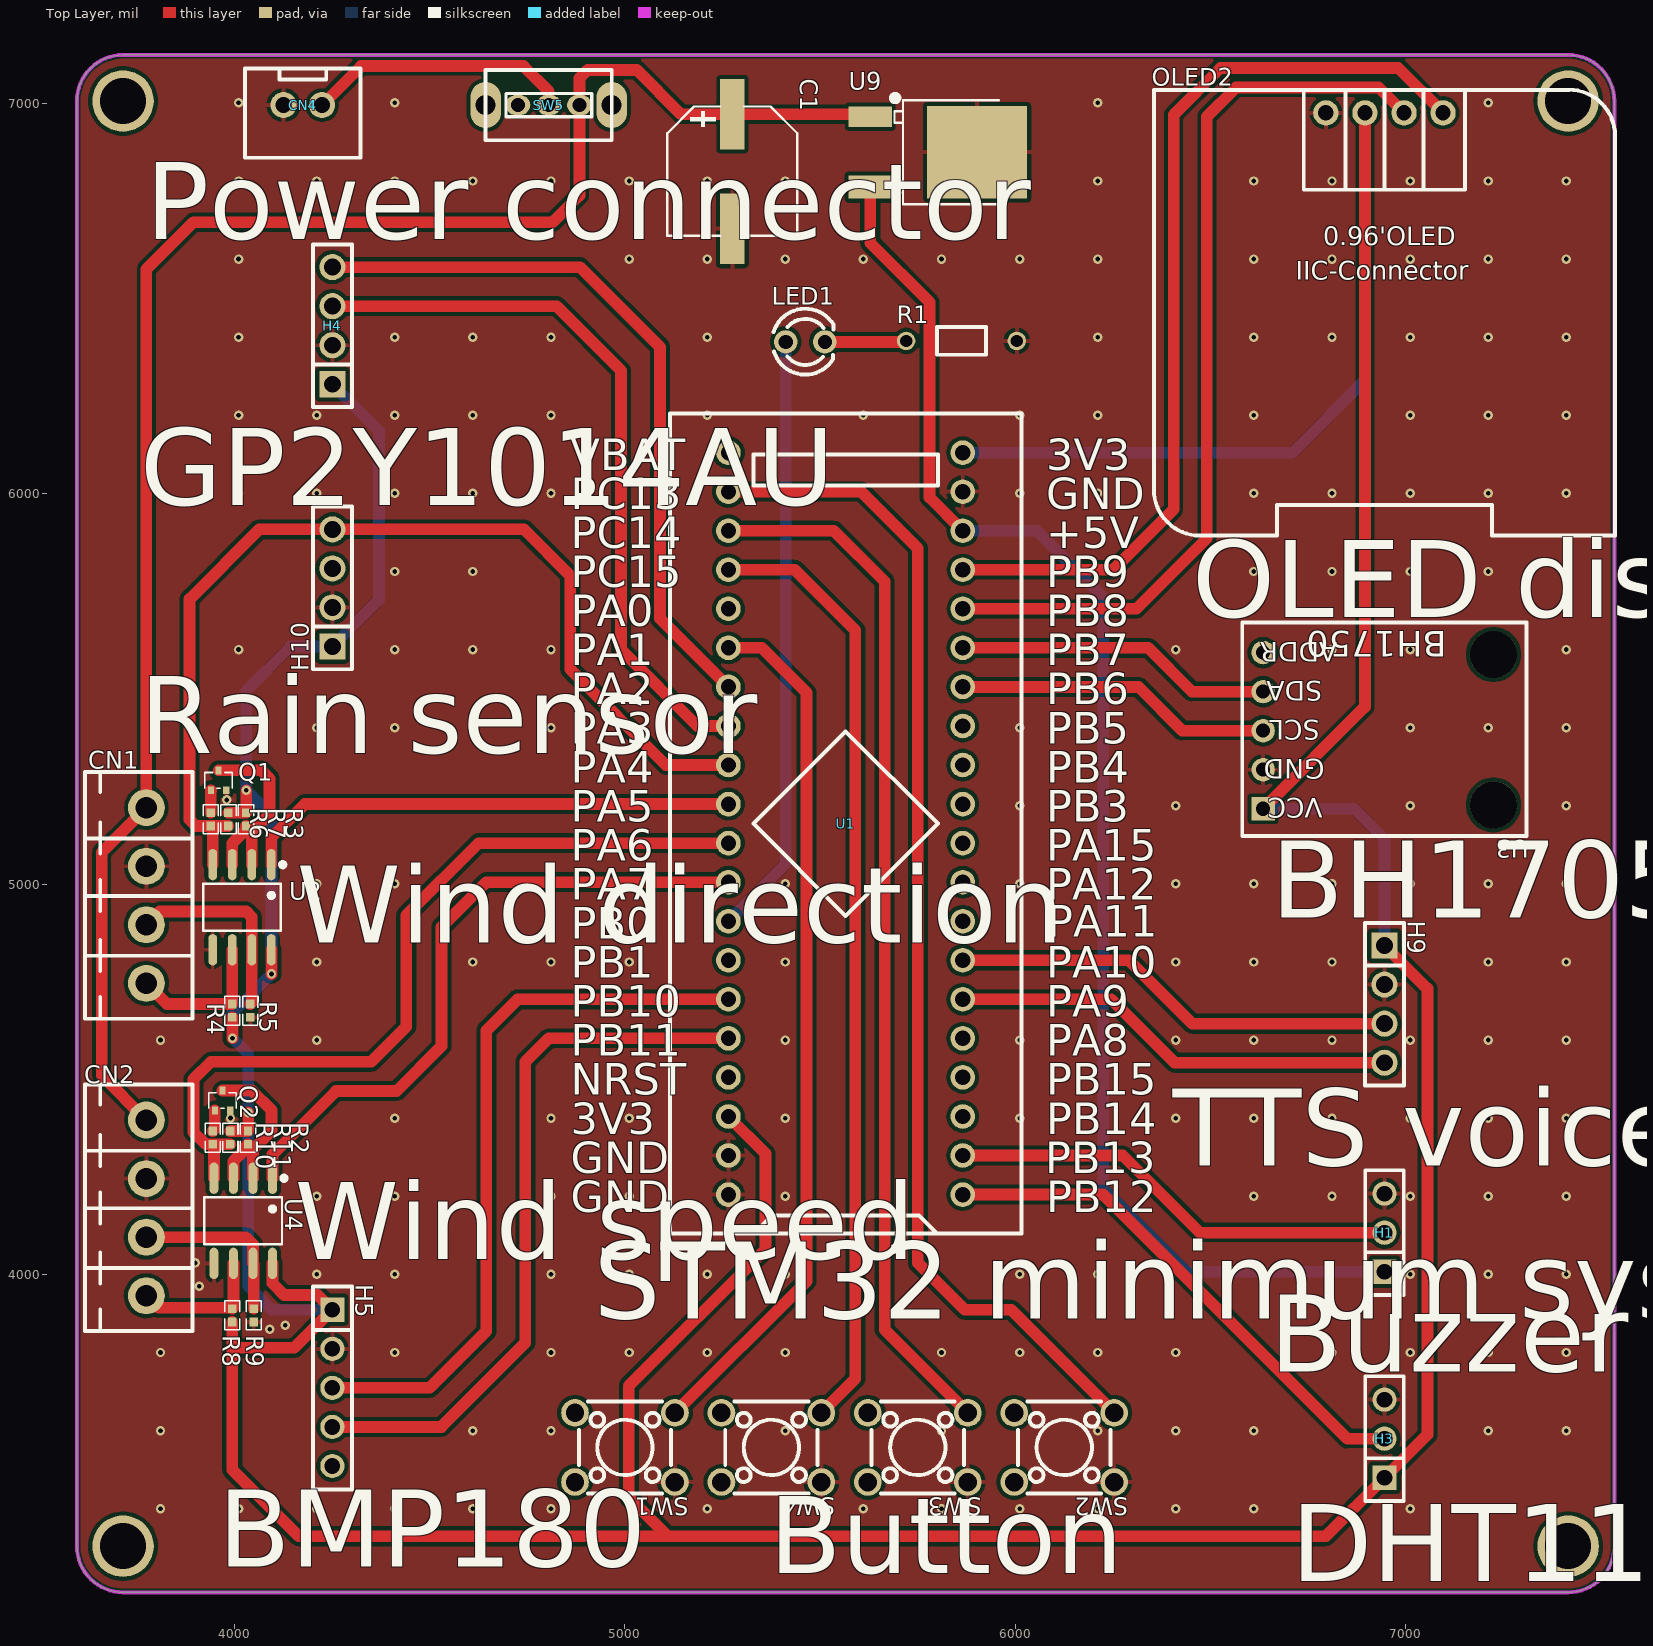
[diagram p0: Top Layer view]
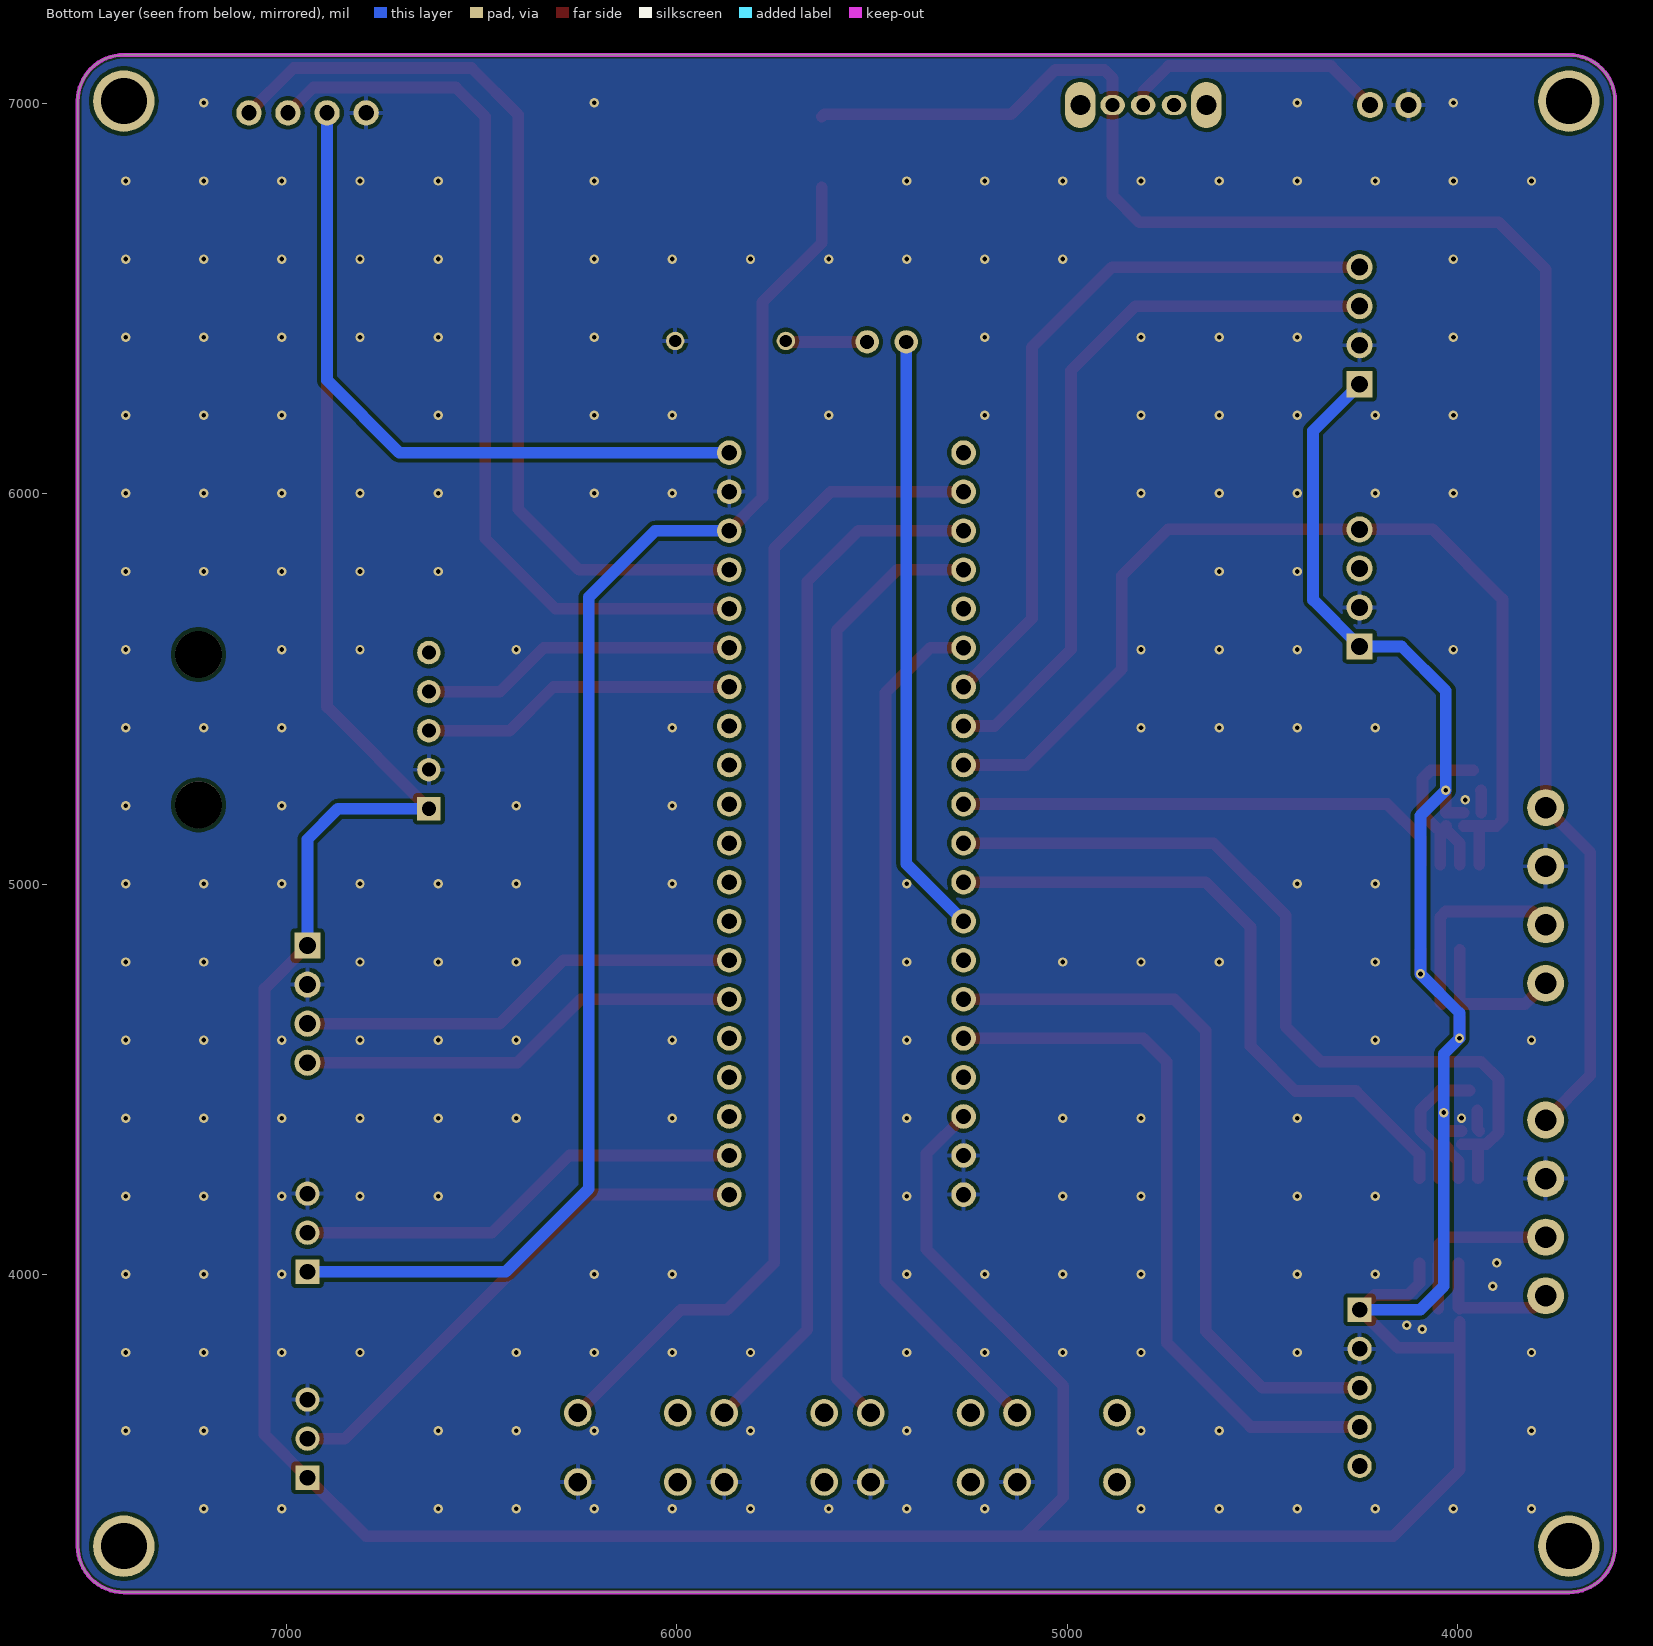
[diagram p1: Bottom Layer view, seen from below]
# Altium PCB MISC51967.pcbdoc
Units mil, origin at the board's own origin, x right, y up, seen from the top; angles counter-clockwise.
Board outline 3937.01 x 3937.01 mil, 2 copper layers (Top Layer, Bottom Layer), stack 62.206 mil thick; 35 components, 48 nets, 160 pads, 207 vias.

## Layer stack, top to bottom
Top Solder Mask Layer: solder mask 0.394, Dk 3.3
Top Layer: signal copper 1.379
Dielectric1: surface 59.449, FR4, Dk 4.5
Bottom Layer: signal copper 1.378
Bottom Solder Mask Layer: solder mask 0.394, Dk 3.3

## Board outline
3714.61,7123.5 ccw(c3714.61,7005.39) 3596.5,7005.39 3596.5,3304.61 ccw(c3714.61,3304.61) 3714.61,3186.5 7415.39,3186.5 ccw(c7415.39,3304.61) 7533.5,3304.61 7533.5,7005.39 ccw(c7415.39,7005.39) 7415.39,7123.5 3714.61,7123.5

## Design rules (kind name [scope] priority, off if disabled: settings)
BoardOutlineClearance copperThickness2oz_1 [All] p2 off: genericclearance=7.99 ignorepadtopadclearanceinfootprint=FALSE except(0: Arc-SplitContinuation Track-SplitContinuation SMDPad-SplitContinuation THPad-SplitContinuation Via-SplitContinuation Fill-SplitContinuation Region-SplitContinuation Poly-SplitContinuation Text-SplitContinuation Hole-SplitContinuation; 5.98: Arc-CutoutEdge Track-CutoutEdge SMDPad-CutoutEdge THPad-CutoutEdge Via-CutoutEdge Text-CutoutEdge; 6.9: Hole-OutlineEdge Hole-CutoutEdge; 10: Poly-OutlineEdge Poly-CutoutEdge; 11.81: Arc-OutlineEdge Track-OutlineEdge SMDPad-OutlineEdge THPad-OutlineEdge Via-OutlineEdge Fill-OutlineEdge Region-OutlineEdge Text-OutlineEdge Fill-CutoutEdge Region-CutoutEdge)
BoardOutlineClearance Plane_innerPlane_1 [All] p4 off: genericclearance=4.02 ignorepadtopadclearanceinfootprint=FALSE except(0: Arc-SplitContinuation Track-SplitContinuation SMDPad-SplitContinuation THPad-SplitContinuation Via-SplitContinuation Fill-SplitContinuation Region-SplitContinuation Poly-SplitContinuation Text-SplitContinuation Hole-SplitContinuation; 5.98: Arc-CutoutEdge Track-CutoutEdge SMDPad-CutoutEdge THPad-CutoutEdge Via-CutoutEdge Text-CutoutEdge; 6.9: Hole-OutlineEdge Hole-CutoutEdge; 10: Poly-OutlineEdge Poly-CutoutEdge; 11.81: Arc-OutlineEdge Track-OutlineEdge SMDPad-OutlineEdge THPad-OutlineEdge Via-OutlineEdge Fill-OutlineEdge Region-OutlineEdge Text-OutlineEdge Fill-CutoutEdge Region-CutoutEdge)
BoardOutlineClearance Copper_copperRegion_1 [All] p6 off: genericclearance=4.02 ignorepadtopadclearanceinfootprint=FALSE except(0: Arc-SplitContinuation Track-SplitContinuation SMDPad-SplitContinuation THPad-SplitContinuation Via-SplitContinuation Fill-SplitContinuation Region-SplitContinuation Poly-SplitContinuation Text-SplitContinuation Hole-SplitContinuation; 5.98: Arc-CutoutEdge Track-CutoutEdge SMDPad-CutoutEdge THPad-CutoutEdge Via-CutoutEdge Text-CutoutEdge; 6.9: Hole-OutlineEdge Hole-CutoutEdge; 10: Poly-OutlineEdge Poly-CutoutEdge; 11.81: Arc-OutlineEdge Track-OutlineEdge SMDPad-OutlineEdge THPad-OutlineEdge Via-OutlineEdge Fill-OutlineEdge Region-OutlineEdge Text-OutlineEdge Fill-CutoutEdge Region-CutoutEdge)
BoardOutlineClearance Copper_copperRegion_copperThickness1oz_1 [All] p8 off: genericclearance=4.02 ignorepadtopadclearanceinfootprint=FALSE except(0: Arc-SplitContinuation Track-SplitContinuation SMDPad-SplitContinuation THPad-SplitContinuation Via-SplitContinuation Fill-SplitContinuation Region-SplitContinuation Poly-SplitContinuation Text-SplitContinuation Hole-SplitContinuation; 5.98: Arc-CutoutEdge Track-CutoutEdge SMDPad-CutoutEdge THPad-CutoutEdge Via-CutoutEdge Text-CutoutEdge; 6.9: Hole-OutlineEdge Hole-CutoutEdge; 10: Poly-OutlineEdge Poly-CutoutEdge; 11.81: Arc-OutlineEdge Track-OutlineEdge SMDPad-OutlineEdge THPad-OutlineEdge Via-OutlineEdge Fill-OutlineEdge Region-OutlineEdge Text-OutlineEdge Fill-CutoutEdge Region-CutoutEdge)
BoardOutlineClearance Copper_copperRegion_Copper_copperRegion_1 [All] p10 off: genericclearance=4.02 ignorepadtopadclearanceinfootprint=FALSE except(0: Arc-SplitContinuation Track-SplitContinuation SMDPad-SplitContinuation THPad-SplitContinuation Via-SplitContinuation Fill-SplitContinuation Region-SplitContinuation Poly-SplitContinuation Text-SplitContinuation Hole-SplitContinuation; 5.98: Arc-CutoutEdge Track-CutoutEdge SMDPad-CutoutEdge THPad-CutoutEdge Via-CutoutEdge Text-CutoutEdge; 6.9: Hole-OutlineEdge Hole-CutoutEdge; 10: Poly-OutlineEdge Poly-CutoutEdge; 11.81: Arc-OutlineEdge Track-OutlineEdge SMDPad-OutlineEdge THPad-OutlineEdge Via-OutlineEdge Fill-OutlineEdge Region-OutlineEdge Text-OutlineEdge Fill-CutoutEdge Region-CutoutEdge)
BoardOutlineClearance copperThickness1oz_1 [All] p12: genericclearance=4.02 ignorepadtopadclearanceinfootprint=FALSE except(0: Arc-SplitContinuation Track-SplitContinuation SMDPad-SplitContinuation THPad-SplitContinuation Via-SplitContinuation Fill-SplitContinuation Region-SplitContinuation Poly-SplitContinuation Text-SplitContinuation Hole-SplitContinuation; 5.98: Arc-CutoutEdge Track-CutoutEdge SMDPad-CutoutEdge THPad-CutoutEdge Via-CutoutEdge Text-CutoutEdge; 6.9: Hole-OutlineEdge Hole-CutoutEdge; 10: Poly-OutlineEdge Poly-CutoutEdge; 11.81: Arc-OutlineEdge Track-OutlineEdge SMDPad-OutlineEdge THPad-OutlineEdge Via-OutlineEdge Fill-OutlineEdge Region-OutlineEdge Text-OutlineEdge Fill-CutoutEdge Region-CutoutEdge)
Clearance copperThickness2oz [All] p1 off: gap=7.99 ignorepadtopadclearanceinfootprint=FALSE except(5.98: SMDPad-Track SMDPad-SMDPad THPad-Track SMDPad-THPad THPad-THPad Track-Via SMDPad-Via THPad-Via Via-Via Fill-SMDPad Region-SMDPad Fill-THPad Region-THPad Fill-Via Region-Via Fill-Fill Fill-Region Region-Region Arc-Track Arc-SMDPad Arc-THPad Arc-Via Fill-Arc Region-Arc Arc-Arc Text-Track SMDPad-Text Text-THPad Text-Via Fill-Text Region-Text Arc-Text Text-Text; 6.9: Hole-Track Hole-SMDPad Hole-THPad Hole-Via Fill-Hole Region-Hole Hole-Arc Hole-Text; 10: Poly-Track Poly-SMDPad Poly-THPad Poly-Via Poly-Fill Poly-Region Poly-Poly Poly-Arc Poly-Text Poly-Hole; 11.81: Fill-Track Region-Track)
Clearance Plane_innerPlane [All] p3 off: gap=4.02 ignorepadtopadclearanceinfootprint=FALSE except(5.98: SMDPad-Track SMDPad-SMDPad THPad-Track SMDPad-THPad THPad-THPad Track-Via SMDPad-Via THPad-Via Via-Via Fill-SMDPad Region-SMDPad Fill-THPad Region-THPad Fill-Via Region-Via Fill-Fill Fill-Region Region-Region Arc-Track Arc-SMDPad Arc-THPad Arc-Via Fill-Arc Region-Arc Arc-Arc Text-Track SMDPad-Text Text-THPad Text-Via Fill-Text Region-Text Arc-Text Text-Text; 6.9: Hole-Track Hole-SMDPad Hole-THPad Hole-Via Fill-Hole Region-Hole Hole-Arc Hole-Text; 10: Poly-Track Poly-SMDPad Poly-THPad Poly-Via Poly-Fill Poly-Region Poly-Poly Poly-Arc Poly-Text Poly-Hole; 11.81: Fill-Track Region-Track)
Clearance Copper_copperRegion [All] p5 off: gap=4.02 ignorepadtopadclearanceinfootprint=FALSE except(5.98: SMDPad-Track SMDPad-SMDPad THPad-Track SMDPad-THPad THPad-THPad Track-Via SMDPad-Via THPad-Via Via-Via Fill-SMDPad Region-SMDPad Fill-THPad Region-THPad Fill-Via Region-Via Fill-Fill Fill-Region Region-Region Arc-Track Arc-SMDPad Arc-THPad Arc-Via Fill-Arc Region-Arc Arc-Arc Text-Track SMDPad-Text Text-THPad Text-Via Fill-Text Region-Text Arc-Text Text-Text; 6.9: Hole-Track Hole-SMDPad Hole-THPad Hole-Via Fill-Hole Region-Hole Hole-Arc Hole-Text; 10: Poly-Track Poly-SMDPad Poly-THPad Poly-Via Poly-Fill Poly-Region Poly-Poly Poly-Arc Poly-Text Poly-Hole; 11.81: Fill-Track Region-Track)
Clearance Copper_copperRegion_copperThickness1oz [All] p7 off: gap=4.02 ignorepadtopadclearanceinfootprint=FALSE except(5.98: SMDPad-Track SMDPad-SMDPad THPad-Track SMDPad-THPad THPad-THPad Track-Via SMDPad-Via THPad-Via Via-Via Fill-SMDPad Region-SMDPad Fill-THPad Region-THPad Fill-Via Region-Via Fill-Fill Fill-Region Region-Region Arc-Track Arc-SMDPad Arc-THPad Arc-Via Fill-Arc Region-Arc Arc-Arc Text-Track SMDPad-Text Text-THPad Text-Via Fill-Text Region-Text Arc-Text Text-Text; 6.9: Hole-Track Hole-SMDPad Hole-THPad Hole-Via Fill-Hole Region-Hole Hole-Arc Hole-Text; 10: Poly-Track Poly-SMDPad Poly-THPad Poly-Via Poly-Fill Poly-Region Poly-Poly Poly-Arc Poly-Text Poly-Hole; 11.81: Fill-Track Region-Track)
Clearance Copper_copperRegion_Copper_copperRegion [All] p9 off: gap=4.02 ignorepadtopadclearanceinfootprint=FALSE except(5.98: SMDPad-Track SMDPad-SMDPad THPad-Track SMDPad-THPad THPad-THPad Track-Via SMDPad-Via THPad-Via Via-Via Fill-SMDPad Region-SMDPad Fill-THPad Region-THPad Fill-Via Region-Via Fill-Fill Fill-Region Region-Region Arc-Track Arc-SMDPad Arc-THPad Arc-Via Fill-Arc Region-Arc Arc-Arc Text-Track SMDPad-Text Text-THPad Text-Via Fill-Text Region-Text Arc-Text Text-Text; 6.9: Hole-Track Hole-SMDPad Hole-THPad Hole-Via Fill-Hole Region-Hole Hole-Arc Hole-Text; 10: Poly-Track Poly-SMDPad Poly-THPad Poly-Via Poly-Fill Poly-Region Poly-Poly Poly-Arc Poly-Text Poly-Hole; 11.81: Fill-Track Region-Track)
Clearance copperThickness1oz [All] p11: gap=4.02 ignorepadtopadclearanceinfootprint=FALSE except(5.98: SMDPad-Track SMDPad-SMDPad THPad-Track SMDPad-THPad THPad-THPad Track-Via SMDPad-Via THPad-Via Via-Via Fill-SMDPad Region-SMDPad Fill-THPad Region-THPad Fill-Via Region-Via Fill-Fill Fill-Region Region-Region Arc-Track Arc-SMDPad Arc-THPad Arc-Via Fill-Arc Region-Arc Arc-Arc Text-Track SMDPad-Text Text-THPad Text-Via Fill-Text Region-Text Arc-Text Text-Text; 6.9: Hole-Track Hole-SMDPad Hole-THPad Hole-Via Fill-Hole Region-Hole Hole-Arc Hole-Text; 10: Poly-Track Poly-SMDPad Poly-THPad Poly-Via Poly-Fill Poly-Region Poly-Poly Poly-Arc Poly-Text Poly-Hole; 11.81: Fill-Track Region-Track)
DiffPairsRouting differentialPair [All] p1: maxlimit=6 minlimit=6 mostfreqgap=6 toplayer_minwidth=5 toplayer_prefwidth=10 toplayer_maxwidth=100 toplayer_mingap=6 toplayer_prefgap=6 toplayer_maxgap=6 bottomlayer_minwidth=5 bottomlayer_prefwidth=10 bottomlayer_maxwidth=100 bottomlayer_mingap=6 bottomlayer_prefgap=6 bottomlayer_maxgap=6 maxuncoupledlength=10
HoleToHoleClearance otherClearance [All] p1: gap=11.81 allowstackedmicrovias=TRUE
Length netLength [All] p1: minlimit=0 maxlimit=0
PasteMaskExpansion pasteMaskExpansion [All] p1: expansion=0
PlaneConnect innerPlane [All] p1: planeconnectstyle=Relief reliefexpansion=20 reliefentries=4 reliefconductorwidth=10 reliefairgap=10
PolygonConnect copperRegion_copperThickness1oz [All] p1 off: connectstyle=Relief reliefconductorwidth=10 reliefentries=4 polygonreliefangle="90 Angle" airgapwidth=10 via.connectstyle=Relief via.reliefconductorwidth=10 via.reliefentries=4 via.polygonreliefangle="90 Angle" via.airgapwidth=10
PolygonConnect copperRegion_Copper_copperRegion [All] p2 off: connectstyle=Relief reliefconductorwidth=10 reliefentries=4 polygonreliefangle="90 Angle" airgapwidth=10 via.connectstyle=Relief via.reliefconductorwidth=10 via.reliefentries=4 via.polygonreliefangle="90 Angle" via.airgapwidth=10
PolygonConnect copperRegion [All] p3: connectstyle=Relief reliefconductorwidth=10 reliefentries=4 polygonreliefangle="90 Angle" airgapwidth=10 via.connectstyle=Relief via.reliefconductorwidth=10 via.reliefentries=4 via.polygonreliefangle="90 Angle" via.airgapwidth=10
RoutingVias viaSize [All] p1: holewidth=12.01 width=24.02 viastyle="Through Hole" minholewidth=11.81 minwidth=19.68 maxholewidth=248.03 maxwidth=393.7
SolderMaskExpansion solderMaskExpansion [IsVia] p1: expansion=-1000 istentingtop=TRUE
SolderMaskExpansion solderMaskExpansion [All] p2: expansion=2 istentingtop=FALSE
Width copperThickness2oz_2 [All] p1 off: maxlimit=100 minlimit=8 preferedwidth=10
Width copperThickness1oz_2 [All] p2: maxlimit=100 minlimit=5 preferedwidth=10

## Components (designator, comment, footprint, x,y, rotation, side; value= is the part's Value field where it differs from the comment)
C1 "" CAP-SMD_BD8.0-L8.3-W8.3-LS9.3-FD 5275,6825 r270 top
CN1 "KF2EDGV-3.81-4P" CONN-TH_4P-P3.81_KF2EDGV-3.81-4P 3774.44,4970.87 r270 top
CN2 "KF2EDGV-3.81-4P" CONN-TH_4P-P3.81_KF2EDGV-3.81-4P 3774.44,4170.87 r270 top
CN4 "XH2.54*2P_through-hole" CONN-TH_2P-P2.50-XH2.54-2P 4175,6995 r0 top
H1 "" HDR-TH_3P-P2.54-V-F 6945,4107.38 r90 top
H3 "" HDR-TH_3P-P2.54-V-F 6945,3579.86 r90 top
H4 "" HDR-TH_4P-P2.54-V-F 4250.79,6430 r90 top
H5 "" HDR-TH_5P-P2.54-V-F 4250.79,3710 r270 top
H9 "" HDR-TH_4P-P2.54-V-F 6945,4692.56 r270 top
H10 "" HDR-TH_4P-P2.54-V-F 4250.79,5758.51 r90 top
LED1 "" LED_TH-3mm 5461.76,6388.51 r0 top
OLED2 "" 0.96OLED_4P 6945,6975 r0 top
Q1 "S8050" SOT-523-3_L1.6-W0.8-P0.50-LS1.6-BR 3959.44,5265.87 r270 top
Q2 "S8050" SOT-523-3_L1.6-W0.8-P0.50-LS1.6-BR 3969.44,4445.87 r270 top
R1 "100" Res_1/8W 5861.76,6388.51 r0 top
R2 "4.7kΩ" R0402ST 4034.44,4350.87 r270 top
R3 "4.7kΩ" R0402ST 4029.44,5165.87 r270 top
R4 "4.7kΩ" R0402ST 3994.44,4675.87 r270 top
R5 "4.7kΩ" R0402ST 4040.63,4675.91 r90 top
R6 "1kΩ" R0402ST 3939.44,5165.87 r270 top
R7 "4.7kΩ" R0402ST 3984.44,5165.87 r270 top
R8 "4.7kΩ" R0402ST 3994.44,3895.87 r270 top
R9 "4.7kΩ" R0402ST 4049.44,3895.87 r90 top
R10 "1kΩ" R0402ST 3944.44,4350.87 r270 top
R11 "4.7kΩ" R0402ST 3989.44,4350.87 r270 top
SW1 "" SW-TH_4P-L6.0-W6.0-P4.50-LS6.5 5000,3557.47 r180 top
SW2 "" SW-TH_4P-L6.0-W6.0-P4.50-LS6.5 6124.9,3557.47 r180 top
SW3 "" SW-TH_4P-L6.0-W6.0-P4.50-LS6.5 5749.93,3557.47 r180 top
SW4 "" SW-TH_4P-L6.0-W6.0-P4.50-LS6.5 5374.97,3557.47 r180 top
SW5 "" 拨动开关 4810,6995 r180 top
U1 "STM32F103C8T6-Card" CONN-TH_L53.3-W22.9_STM32F103C8T6-CARD 5565,5155 r90 top
U2 "XL3485" SOP-8_L5.0-W4.0-P1.27-LS6.0-BL 4019.44,4940.87 r180 top
U3 "" BH1750光照传感器 6894.17,5402.97 r180 top
U4 "XL3485" SOP-8_L5.0-W4.0-P1.27-LS6.0-BL 4022.43,4137.84 r180 top
U9 "L78M05ABDT-TR" TO-252-2_L6.5-W6.1-P4.58-LS10.0-TL 5765,6875 r0 top

## Footprints (in the part's own frame and the unit in brackets; to place one, negate y for a bottom-side part, rotate by r counter-clockwise, add the part's x,y. Pads: shape width x height; smd on the part's side, far side on the other; paste and mask are expansions set on the pad)
0.96OLED_4P [mm]
  round 1.65 hole 1 copper offset 0,0: 1(-3.81,-0.001) 2(-1.27,0.002) 3(1.27,0.002) 4(3.81,0.002)
  silkscreen extent -15,-27.5 15,1.5
BH1750光照传感器 [mil]
  rect 60x60 hole 36: 1(260,210)
  round 60 hole 36: 2(260,110) 3(260,10) 4(260,-90) 5(260,-190)
  round 120 hole 120 unplated: ""(-330,-185) ""(-330,200)
  silkscreen extent -415,-267 313,280
CAP-SMD_BD8.0-L8.3-W8.3-LS9.3-FD [mil]
  rect 181.1x63 smd paste+0 mask+2: 1(-146.6,0) 2(146.6,0)
  silkscreen extent -166,-166 164,166
CONN-TH_2P-P2.50-XH2.54-2P [mm]
  round 1.7 hole 1.05 paste+0 mask+0.05: 1(1.25,0) 2(-1.25,0)
  silkscreen extent -3.75,-3.42 3.75,2.37
CONN-TH_4P-P3.81_KF2EDGV-3.81-4P [mm]
  round 2.4 hole 1.4: 1(-5.715,0) 2(-1.905,0) 3(1.905,0) 4(5.715,0)
  silkscreen extent -8.02,-4 8.02,3
CONN-TH_L53.3-W22.9_STM32F103C8T6-CARD [mm]
  round 1.6 hole 1: 1(-24.13,-7.62) 2(-21.59,-7.62) 3(-19.05,-7.62) 4(-16.51,-7.62) 5(-13.97,-7.62) 6(-11.43,-7.62) 7(-8.89,-7.62) 8(-6.35,-7.62) 9(-3.81,-7.62) 10(-1.27,-7.62) 11(1.27,-7.62) 12(3.81,-7.62) 13(6.35,-7.62) 14(8.89,-7.62) 15(11.43,-7.62) 16(13.97,-7.62) 17(16.51,-7.62) 18(19.05,-7.62) 19(21.59,-7.62) 20(24.13,-7.62) 21(24.13,7.62) 22(21.59,7.62) 23(19.05,7.62) 24(16.51,7.62) 25(13.97,7.62) 26(11.43,7.62) 27(8.89,7.62) 28(6.35,7.62) 29(3.81,7.62) 30(1.27,7.62) 31(-1.27,7.62) 32(-3.81,7.62) 33(-6.35,7.62) 34(-8.89,7.62) 35(-11.43,7.62) 36(-13.97,7.62) 37(-16.51,7.62) 38(-19.05,7.62) 39(-21.59,7.62) 40(-24.13,7.62)
  silkscreen extent -26.67,-11.43 26.67,11.43
HDR-TH_3P-P2.54-V-F [mil]
  rect 62x62 hole 40.16: 1(-100,0)
  round 62 hole 40.16: 2(0,0) 3(100,0)
  silkscreen extent -160,-49 160,49
HDR-TH_4P-P2.54-V-F [mm]
  rect 1.7x1.7 hole 1.1: 1(-3.81,0)
  round 1.7 hole 1.1: 2(-1.27,0) 3(1.27,0) 4(3.81,0)
  silkscreen extent -5.29,-1.27 5.29,1.27
HDR-TH_5P-P2.54-V-F [mil]
  rect 62x62 hole 40.16: 1(-200,0)
  round 62 hole 40.16: 2(-100,0) 3(0,0) 4(100,0) 5(200,0)
  silkscreen extent -260,-50 260,50
LED_TH-3mm [mil]
  round 60 hole 36 paste+0 mask+2: 1(-50,0) 2(50,0)
  silkscreen extent -81,-84 72,85
R0402ST [mm]
  rect 0.566x0.54 smd paste-100 mask+0.051: 1(-0.433,0) 2(0.433,0)
  silkscreen extent -0.94,-0.5 0.94,0.5
Res_1/8W [mil]
  round 47.2 hole 31.5 paste+0 mask+2: 1(-141.7,2.48) 2(141.7,2.48)
  silkscreen extent -63,-33 63,38
SOP-8_L5.0-W4.0-P1.27-LS6.0-BL [mil]
  oval 22.6x80.14 smd: 1(-75,-108.97) 2(-25,-108.97) 3(25,-108.97) 4(75,-108.97) 5(75,108.97) 6(25,108.97) 7(-25,108.97) 8(-75,108.97)
  silkscreen extent -110,-115 99,60
SOT-523-3_L1.6-W0.8-P0.50-LS1.6-BR [mm]
  rect 0.51x0.4 smd paste+0 mask+0.05: 1(0.645,-0.5) 2(0.645,0.5) 3(-0.645,0)
  silkscreen extent -0.51,-0.89 0.51,0.89
SW-TH_4P-L6.0-W6.0-P4.50-LS6.5 [mm]
  round 1.8 hole 1.2: 1(-3.25,2.25) 2(3.25,2.25) 3(-3.25,-2.25) 4(3.25,-2.25)
  silkscreen extent -3,-3 3,3
TO-252-2_L6.5-W6.1-P4.58-LS10.0-TL [mm]
  rect 2.8x1.35 smd paste+0 mask+0.051: 1(-3.475,2.29)
  rect 2.8x1.5 smd paste+0 mask+0.051: 3(-3.475,-2.29)
  rect 6.5x6 smd paste+0 mask+0.051: 4(3.475,-0.017)
  silkscreen extent -2.06,-3.39 4.9,3.7
拨动开关 [mil]
  oval 63x51.2 hole 35.4 paste+0 mask+2: 1(-73.4,0) 2(5,0) 3(84,0)
  oval 78.7x118.1 hole 51.2 paste+0 mask+2: 4(166.7,0) 5(-156.1,0)
  silkscreen extent -156,-90 167,90

## Free pads (board coordinates)
  round 157.48 hole 118.11: 1(3714.61,7005.39) 1(3714.61,3304.61) 1(7415.39,7005.39) 1(7415.39,3304.61)

## Via types
v1: diameter 24.02, hole 12, Top Layer to Bottom Layer, 207 vias

## Nets (pads, with @x,y where several pads share a name; then routed paths per layer and width w, separated by ;. In a path a pad name is that pad's centre, name@x,y a point inside that pad or via, vN(x,y) a via of type N, cw(c..) or ccw(c..) an arc to the next point about the centre after c; other vN are vias at no path point)
$1N17118: CN4.1 SW5.2 | length 684.1
  Top Layer w30: CN4.1 4324.22,7095 4740,7095 4805,7030 SW5.2
$1N17160: LED1.2 R1.1 | length 209.3
  Top Layer w30: LED1.2 5717.58,6388.51 R1.1
$1N17193: CN1.4 R4.1 U2.6 | length 380.9
  Top Layer w30: CN1.4 3827.4,4692.91 R4.1 U2.6
$1N17195: CN1.3 R5.2 U2.7 | length 514.3
  Top Layer w30: CN1.3 3808.57,4930 4030,4930 4044.44,4915.56 U2.7 4044.44,4696.76 R5.2
$1N17201: Q1.3 R3.2 U2.2 U2.3 | length 504.4
  Top Layer w30: Q1.3 4068.74,5291.26 4090,5270 4090,5180 4050.15,5140.15 R3.2@4038.12,5140.15 ; U2.3 3994.44,5104.44 4025,5135 ; R3.2 R3.2@4038.12,5140.15 ; 4035,5130 4035,5137.02 R3.2@4038.12,5140.15 ; 4041.64,5136.64 R3.2@4038.12,5140.15 ; U2.2 4044.44,5130
$1N17209: Q1.1 R6.1 | length 57.7
  Top Layer w30: R6.1 3939.44,5240.16 Q1.1
$1N17234: CN2.4 R8.1 U4.6 | length 350.9
  Top Layer w30: CN2.4 3805.31,3915 3992.35,3915 R8.1 3997.43,3915.89 U4.6
$1N17235: CN2.3 R9.2 U4.7 | length 446.1
  Top Layer w30: CN2.3 4029.13,4095.87 4047.43,4077.57 U4.7 4049.44,4026.86 R9.2
$1N17238: Q2.3 R2.2 U4.2 U4.3 | length 461.1
  Top Layer w30: Q2.3 4045,4471.26 4095,4421.26 4095,4368.42 4047.43,4320.85 ; U4.3 3997.43,4290.37 4023.46,4316.4 4023.46,4322.85 R2.2 4047.43,4320.85 ; U4.2 4047.43,4320.85
$1N17241: Q2.1 R10.1 | length 54.8
  Top Layer w30: R10.1 3949.76,4373.22 Q2.1
+5V: H1.1 U1.18 U9.3 | length 3731.4
  Top Layer w30: U9.3 5628.19,6641.81 5780,6490 5780,5990 U1.18
  Bottom Layer w30: U1.18 6055,5905 6225,5735 6225,4220 6437.62,4007.38 H1.1
+12V: C1.1 CN1.1 CN2.1 SW5.1 U9.1 | length 4564
  Top Layer w30: CN2.1 3660,4510.31 3660,5081.43 CN1.1 3774.44,6574.44 3895,6695 4815,6695 4883.4,6763.4 SW5.1 4883.4,7063.4 4905,7085 5030,7085 5143.4,6971.6 C1.1 5621.74,6971.6 U9.1
GND: C1.2 CN1.2 CN2.2 CN4.2 H1.3 H3.3 H4.2 H5.2 H9.2 H10.2 OLED2.1 Q1.2 Q2.2 R1.2 R5.1 R9.1 SW1.1 SW2.1 SW3.1 SW4.1 U1.19 U1.39 U1.40 U2.5 U3.2 U4.5 U9.4
  other v1: 3810.6,3400.6 4010.6,3400.6 4210.6,3400.6 4410.6,3400.6 4610.6,3400.6 4810.6,3400.6 5210.6,3400.6 5410.6,3400.6 5610.6,3400.6 5810.6,3400.6 6010.6,3400.6 6210.6,3400.6 6410.6,3400.6 6610.6,3400.6 7010.6,3400.6 7210.6,3400.6 3810.6,3600.6 4610.6,3600.6 4810.6,3600.6 5410.6,3600.6 5810.6,3600.6 6210.6,3600.6 6410.6,3600.6 6610.6,3600.6 7210.6,3600.6 7410.6,3600.6 3810.6,3800.6 4410.6,3800.6 4810.6,3800.6 5010.6,3800.6 5210.6,3800.6 5410.6,3800.6 5810.6,3800.6 6010.6,3800.6 6210.6,3800.6 6410.6,3800.6 6810.6,3800.6 7010.6,3800.6 7210.6,3800.6 7410.6,3800.6 4090,3860 4130,3870 3910,3970 4210.6,4000.6 4410.6,4000.6 4810.6,4000.6 5010.6,4000.6 5210.6,4000.6 5410.6,4000.6 6010.6,4000.6 6210.6,4000.6 7010.6,4000.6 7210.6,4000.6 7410.6,4000.6 3900,4030 4210.6,4200.6 4410.6,4200.6 4810.6,4200.6 5010.6,4200.6 5410.6,4200.6 6610.6,4200.6 6810.6,4200.6 7010.6,4200.6 7210.6,4200.6 7410.6,4200.6 3990,4400.9 4410.6,4400.6 4810.6,4400.6 5010.6,4400.6 5410.6,4400.6 6010.6,4400.6 6410.6,4400.6 6610.6,4400.6 6810.6,4400.6 7010.6,4400.6 7210.6,4400.6 7410.6,4400.6 3810.6,4600.6 4210.6,4600.6 5410.6,4600.6 6010.6,4600.6 6410.6,4600.6 6610.6,4600.6 6810.6,4600.6 7010.6,4600.6 7210.6,4600.6 7410.6,4600.6 4210.6,4800.6 4610.6,4800.6 4810.6,4800.6 5010.6,4800.6 5410.6,4800.6 6410.6,4800.6 6610.6,4800.6 6810.6,4800.6 7210.6,4800.6 7410.6,4800.6 4210.6,5000.6 4410.6,5000.6 5410.6,5000.6 6010.6,5000.6 6410.6,5000.6 6610.6,5000.6 6810.6,5000.6 7010.6,5000.6 7210.6,5000.6 7410.6,5000.6 6010.6,5200.6 6410.6,5200.6 7010.6,5200.6 7410.6,5200.6 3979.92,5215.59 4210.6,5400.6 4410.6,5400.6 4610.6,5400.6 4810.6,5400.6 6010.6,5400.6 7010.6,5400.6 7210.6,5400.6 7410.6,5400.6 4010.6,5600.6 4410.6,5600.6 4610.6,5600.6 4810.6,5600.6 6410.6,5600.6 6810.6,5600.6 7010.6,5600.6 7410.6,5600.6 4410.6,5800.6 4610.6,5800.6 6610.6,5800.6 6810.6,5800.6 7010.6,5800.6 7210.6,5800.6 7410.6,5800.6 4010.6,6000.6 4210.6,6000.6 4410.6,6000.6 4610.6,6000.6 4810.6,6000.6 6010.6,6000.6 6210.6,6000.6 6610.6,6000.6 6810.6,6000.6 7010.6,6000.6 7210.6,6000.6 7410.6,6000.6 4010.6,6200.6 4210.6,6200.6 4410.6,6200.6 4610.6,6200.6 4810.6,6200.6 5210.6,6200.6 5610.6,6200.6 6010.6,6200.6 6210.6,6200.6 6610.6,6200.6 7010.6,6200.6 7210.6,6200.6 7410.6,6200.6 4010.6,6400.6 4410.6,6400.6 4610.6,6400.6 4810.6,6400.6 5210.6,6400.6 6210.6,6400.6 6610.6,6400.6 6810.6,6400.6 7010.6,6400.6 7210.6,6400.6 7410.6,6400.6 4010.6,6600.6 5010.6,6600.6 5210.6,6600.6 5410.6,6600.6 5610.6,6600.6 5810.6,6600.6 6010.6,6600.6 6210.6,6600.6 6610.6,6600.6 6810.6,6600.6 7010.6,6600.6 7210.6,6600.6 7410.6,6600.6 3810.6,6800.6 4010.6,6800.6 4210.6,6800.6 4410.6,6800.6 4610.6,6800.6 4810.6,6800.6 5010.6,6800.6 5210.6,6800.6 5410.6,6800.6 6210.6,6800.6 6610.6,6800.6 6810.6,6800.6 7010.6,6800.6 7210.6,6800.6 7410.6,6800.6 4010.6,7000.6 4410.6,7000.6 6210.6,7000.6 7210.6,7000.6
NRST: U1.37
PA0: U1.25
PA1: SW1.3 U1.26 | length 2231.2
  Top Layer w30: SW1.3 5465,3983.1 5465,5490 5350,5605 U1.26
PA2: H4.4 U1.27 | length 1866.6
  Top Layer w30: H4.4 4885,6580 5090,6375 5090,5680 U1.27
PA3: H4.3 U1.28 | length 1878.3
  Top Layer w30: H4.3 4825,6480 4990,6315 4990,5600 5185,5405 U1.28
PA4: H10.4 R6.2 R7.2 U1.29 U2.4 | length 2616.7
  Top Layer w30: U2.4 3944.44,5143.83 R6.2 ; R7.2 R6.2 ; U1.29 5105,5305 4860,5550 4860,5790 4741.49,5908.51 H10.4 4063.51,5908.51 3885,5730 3885,5165 3901.17,5148.83 R6.2
PA5: U1.30 U2.1 | length 1275.6
  Top Layer w30: U2.1 4094.44,5119.44 4180,5205 U1.30
PA6: R10.2 R11.2 U1.31 U4.4 | length 2118.2
  Top Layer w30: U4.4 3947.43,4330.85 R10.2 ; R11.2 R10.2 ; U1.31 4625,5105 4440,4920 4440,4635 4350,4545 3940,4545 3895,4500 3895,4365 3926.17,4333.83 R10.2
PA7: U1.32 U4.1 | length 1695.8
  Top Layer w30: U4.1 4097.43,4307.43 4260,4470 4415,4470 4530,4585 4530,4890 4645,5005 U1.32
PA8: U1.5
PA9: H9.4 U1.6 | length 1147.3
  Top Layer w30: U1.6 6245,4705 6407.44,4542.56 H9.4
PA10: H9.3 U1.7 | length 1147.3
  Top Layer w30: U1.7 6290,4805 6452.44,4642.56 H9.3
PA11: U1.8
PA12: U1.9
PA15: U1.10
PB0: LED1.1 U1.33 | length 1544.3
  Bottom Layer w30: U1.33 5411.76,5051.76 LED1.1
PB1: U1.34
PB3: U1.11
PB4: U1.12
PB5: U1.13
PB6: U1.14 U3.3 | length 815.6
  Top Layer w30: U1.14 6315,5505 6427.03,5392.97 U3.3
PB7: U1.15 U3.4 | length 815.6
  Top Layer w30: U1.15 6340,5605 6452.03,5492.97 U3.4
PB8: OLED2.3 U1.16 | length 2342.5
  Top Layer w30: U1.16 6310,5705 6490,5885 6490,6965 6565,7040 6930.05,7040 OLED2.3@6995,6975.05
PB9: OLED2.4 U1.17 | length 2401.5
  Top Layer w30: U1.17 6250,5805 6405,5960 6405,6970 6525,7090 6980.05,7090 OLED2.4@7095,6975.05
PB10: H5.3 U1.35 | length 1877.4
  Top Layer w30: H5.3 4500,3710 4645,3855 4645,4625 4725,4705 U1.35
PB11: H5.4 U1.36 | length 1848.1
  Top Layer w30: H5.4 4530,3610 4745,3825 4745,4545 4805,4605 U1.36
PB12: H3.2 U1.1 | length 1338.9
  Top Layer w30: U1.1 6225,4205 6850.14,3579.86 H3.2
PB13: H1.2 U1.2 | length 1161.9
  Top Layer w30: U1.2 6275,4305 6472.62,4107.38 H1.2
PB14: U1.3
PB15: U1.4
PC13: SW2.3 U1.22 | length 3036.9
  Top Layer w30: U1.22 5605,6005 5750,5860 5750,4030 5870,3910 5988.9,3910 SW2.3@6252.85,3646.05
PC14: SW3.3 U1.23 | length 2671
  Top Layer w30: U1.23 5535,5905 5665,5775 5665,3858.93 SW3.3
PC15: SW4.3 U1.24 | length 2429.2
  Top Layer w30: U1.24 5435,5805 5590,5650 5590,3733.13 SW4.3
VBAT: U1.21
VCC: H3.1 H4.1 H5.1 H9.1 H10.1 OLED2.2 R2.1 R3.1 R4.2 R7.1 R8.2 R11.1 U1.20 U1.38 U2.8 U3.1 U4.8 | length 14242.3
  Top Layer w30: R7.1 R3.1 4030,5183.47 v1(4030,5240) ; R11.1 R2.1 4035,4368.47 v1(4035,4415) ; R8.2 3994.44,3812.45 ; R4.2 3995,4658.27 v1(3995,4605) ; U2.8 4095,4831.34 v1(4095,4770) ; U4.8 4097.43,3977.57 4127.43,3947.57 4213.21,3947.57 H5.1 4153.24,3812.45 3994.44,3812.45 ; U1.38 5360,4310 5360,4065 5010,3715 5010,3430 5110,3330 ; U3.1 6895,5453.8 OLED2.2@6895,6975.05 ; H9.1 7055,4732.55 7055,3589.87 H3.1 6795.13,3330 5110,3330 ; 3994.44,3812.45 3994.44,3500.56 4165,3330 5110,3330
  Bottom Layer w30: H5.1 4095,3910 4035,3970 v1(4035,4415) 4035,4565 v1(3995,4605) 3995,4670 v1(4095,4770) 4095,5175 v1(4030,5240) 4030,5495 4143.51,5608.51 H10.1 4370,5727.72 4370,6160.79 H4.1 ; U1.20 6710,6105 6895,6290 OLED2.2@6895,6975.05 ; U3.1 6867.03,5192.97 6945,5115 H9.1
pads on no net: H5.5 H10.3 SW1.2 SW1.4 SW2.2 SW2.4 SW3.2 SW3.4 SW4.2 SW4.4 SW5.3 SW5.4 SW5.5 U3. U3.5

## Polygon pours and split planes (outlines as drawn)
GND on Bottom Layer (solid, remove dead copper, pour order 2): 3525,7245 3525,3080 7700,3080 7700,7245
GND on Top Layer (solid, remove dead copper, pour order 2): 3000,7415 3000,3000 7930,3000 7930,7415

## Keep-outs
Board Outline Layer:
  the board outline again, w10

## Silkscreen, mask and mechanical layers (free items; w line width, h text height)
Top Silkscreen Layer:
  text "Power connector" at 3772.87,6651.57 h196.85
  text "VBAT" at 4860.95,6060 h80
  text "3V3" at 6079.16,6060 h80
  text "GP2Y1014AU" at 3758.96,5970 h196.85
  text "PC13" at 4860.95,5960 h80
  text "GND" at 6079.16,5960 h80
  text "PC14" at 4860.95,5860 h80
  text "+5V" at 6079.16,5860 h80
  text "PC15" at 4860.95,5760 h80
  text "PB9" at 6079.16,5760 h80
  text "OLED display" at 6453.02,5682.86 h196.85
  text "PA0" at 4860.95,5660 h80
  text "PB8" at 6079.16,5660 h80
  text "PA1" at 4860.95,5560 h80
  text "PB7" at 6079.16,5560 h80
  text "PA2" at 4860.95,5460 h80
  text "PB6" at 6079.16,5460 h80
  text "PA3" at 4860.95,5360 h80
  text "PB5" at 6079.16,5360 h80
  text "Rain sensor" at 3757.32,5335 h196.85
  text "PA4" at 4860.95,5260 h80
  text "PB4" at 6079.16,5260 h80
  text "PA5" at 4860.95,5160 h80
  text "PB3" at 6079.16,5160 h80
  text "PA6" at 4860.95,5060 h80
  text "PA15" at 6079.16,5060 h80
  text "PA7" at 4860.95,4960 h80
  text "PA12" at 6079.16,4960 h80
  text "BH1705" at 6654.49,4913.47 h196.85
  text "PA11" at 6080.95,4865 h80
  text "PB0" at 4860.95,4860 h80
  text "Wind direction" at 4160,4850 h196.85
  text "PB1" at 4860.95,4760 h80
  text "PA10" at 6079.16,4760 h80
  text "PB10" at 4860.95,4660 h80
  text "PA9" at 6079.16,4660 h80
  text "PB11" at 4860.95,4560 h80
  text "PA8" at 6079.16,4560 h80
  text "NRST" at 4860.95,4460 h80
  text "PB15" at 6079.16,4460 h80
  text "3V3" at 4860.95,4360 h80
  text "PB14" at 6079.16,4360 h80
  text "TTS voice module" at 6402.8,4279.27 h196.85
  text "GND" at 4860.95,4260 h80
  text "PB13" at 6075.95,4260 h80
  text "GND" at 4860.95,4160 h80
  text "PB12" at 6079.16,4160 h80
  text "Wind speed" at 4155,4040 h196.85
  text "STM32 minimum system" at 4919.45,3886.57 h196.85
  text "Buzzer" at 6651.81,3751.76 h196.85
  text "BMP180" at 3959.09,3251.57 h196.85
  text "Button" at 5370,3235 h196.85
  text "DHT11" at 6706.39,3215 h196.85